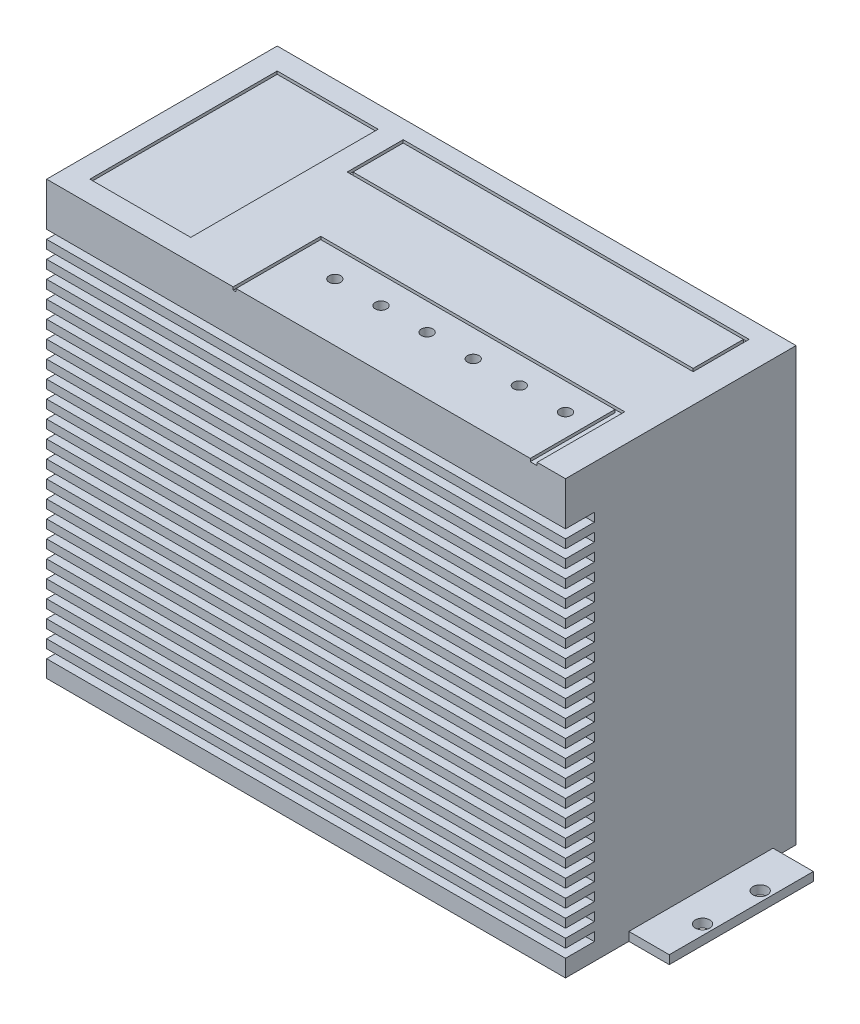
from build123d import *

# Parameters (mm, degrees)
SKETCH_1_W          = 180
SKETCH_1_H          = 150
EXTRUDE_1_DEPTH     = 40
CUT_EXTRUDE_1_REACH = 201.06
SKETCH_2_W          = 10
SKETCH_2_H          = 3
SKETCH_3_W          = 35
SKETCH_3_H          = 65
CUT_EXTRUDE_2_DEPTH = 1
SKETCH_4_W          = 120
SKETCH_4_H          = 19.42574098
SKETCH_4_W_2        = 118
SKETCH_4_H_2        = 17.42574098
CUT_EXTRUDE_3_DEPTH = 1
SKETCH_5_W          = 14
SKETCH_5_H          = 50
SKETCH_5_R          = 2.5
EXTRUDE_2_DEPTH     = 3
SKETCH_6_R          = 2
CUT_EXTRUDE_4_DEPTH = 4
CUT_EXTRUDE_5_DEPTH = 1


with BuildPart() as part:
    # 草图1 → 凸台-拉伸1 (new, symmetric)
    with BuildSketch(Plane.XY):
        Rectangle(SKETCH_1_W, SKETCH_1_H)
    extrude(amount=EXTRUDE_1_DEPTH, both=True)

    # 草图2 → 切除-拉伸1 (cut, up to next)
    with BuildSketch(Plane.ZY.offset(90), mode=Mode.PRIVATE) as cut_extrude_1_sk1:
        with Locations((35, 58.423056781)):
            Rectangle(SKETCH_2_W, SKETCH_2_H)
    cut_extrude_1_tool1 = extrude(cut_extrude_1_sk1.sketch, amount=-CUT_EXTRUDE_1_REACH, mode=Mode.PRIVATE) & part.part
    # 草图2 → 切除-拉伸1 (cut, up to next)
    with BuildSketch(Plane.ZY.offset(90), mode=Mode.PRIVATE) as cut_extrude_1_sk2:
        with Locations((35, 52.423056781)):
            Rectangle(SKETCH_2_W, SKETCH_2_H)
    cut_extrude_1_tool2 = extrude(cut_extrude_1_sk2.sketch, amount=-CUT_EXTRUDE_1_REACH, mode=Mode.PRIVATE) & part.part
    # 草图2 → 切除-拉伸1 (cut, up to next)
    with BuildSketch(Plane.ZY.offset(90), mode=Mode.PRIVATE) as cut_extrude_1_sk3:
        with Locations((35, 46.423056781)):
            Rectangle(SKETCH_2_W, SKETCH_2_H)
    cut_extrude_1_tool3 = extrude(cut_extrude_1_sk3.sketch, amount=-CUT_EXTRUDE_1_REACH, mode=Mode.PRIVATE) & part.part
    # 草图2 → 切除-拉伸1 (cut, up to next)
    with BuildSketch(Plane.ZY.offset(90), mode=Mode.PRIVATE) as cut_extrude_1_sk4:
        with Locations((35, 40.423056781)):
            Rectangle(SKETCH_2_W, SKETCH_2_H)
    cut_extrude_1_tool4 = extrude(cut_extrude_1_sk4.sketch, amount=-CUT_EXTRUDE_1_REACH, mode=Mode.PRIVATE) & part.part
    # 草图2 → 切除-拉伸1 (cut, up to next)
    with BuildSketch(Plane.ZY.offset(90), mode=Mode.PRIVATE) as cut_extrude_1_sk5:
        with Locations((35, 34.423056781)):
            Rectangle(SKETCH_2_W, SKETCH_2_H)
    cut_extrude_1_tool5 = extrude(cut_extrude_1_sk5.sketch, amount=-CUT_EXTRUDE_1_REACH, mode=Mode.PRIVATE) & part.part
    # 草图2 → 切除-拉伸1 (cut, up to next)
    with BuildSketch(Plane.ZY.offset(90), mode=Mode.PRIVATE) as cut_extrude_1_sk6:
        with Locations((35, 28.423056781)):
            Rectangle(SKETCH_2_W, SKETCH_2_H)
    cut_extrude_1_tool6 = extrude(cut_extrude_1_sk6.sketch, amount=-CUT_EXTRUDE_1_REACH, mode=Mode.PRIVATE) & part.part
    # 草图2 → 切除-拉伸1 (cut, up to next)
    with BuildSketch(Plane.ZY.offset(90), mode=Mode.PRIVATE) as cut_extrude_1_sk7:
        with Locations((35, 22.423056781)):
            Rectangle(SKETCH_2_W, SKETCH_2_H)
    cut_extrude_1_tool7 = extrude(cut_extrude_1_sk7.sketch, amount=-CUT_EXTRUDE_1_REACH, mode=Mode.PRIVATE) & part.part
    # 草图2 → 切除-拉伸1 (cut, up to next)
    with BuildSketch(Plane.ZY.offset(90), mode=Mode.PRIVATE) as cut_extrude_1_sk8:
        with Locations((35, 16.423056781)):
            Rectangle(SKETCH_2_W, SKETCH_2_H)
    cut_extrude_1_tool8 = extrude(cut_extrude_1_sk8.sketch, amount=-CUT_EXTRUDE_1_REACH, mode=Mode.PRIVATE) & part.part
    # 草图2 → 切除-拉伸1 (cut, up to next)
    with BuildSketch(Plane.ZY.offset(90), mode=Mode.PRIVATE) as cut_extrude_1_sk9:
        with Locations((35, 10.423056781)):
            Rectangle(SKETCH_2_W, SKETCH_2_H)
    cut_extrude_1_tool9 = extrude(cut_extrude_1_sk9.sketch, amount=-CUT_EXTRUDE_1_REACH, mode=Mode.PRIVATE) & part.part
    # 草图2 → 切除-拉伸1 (cut, up to next)
    with BuildSketch(Plane.ZY.offset(90), mode=Mode.PRIVATE) as cut_extrude_1_sk10:
        with Locations((35, 4.423056781)):
            Rectangle(SKETCH_2_W, SKETCH_2_H)
    cut_extrude_1_tool10 = extrude(cut_extrude_1_sk10.sketch, amount=-CUT_EXTRUDE_1_REACH, mode=Mode.PRIVATE) & part.part
    # 草图2 → 切除-拉伸1 (cut, up to next)
    with BuildSketch(Plane.ZY.offset(90), mode=Mode.PRIVATE) as cut_extrude_1_sk11:
        with Locations((35, -1.576943219)):
            Rectangle(SKETCH_2_W, SKETCH_2_H)
    cut_extrude_1_tool11 = extrude(cut_extrude_1_sk11.sketch, amount=-CUT_EXTRUDE_1_REACH, mode=Mode.PRIVATE) & part.part
    # 草图2 → 切除-拉伸1 (cut, up to next)
    with BuildSketch(Plane.ZY.offset(90), mode=Mode.PRIVATE) as cut_extrude_1_sk12:
        with Locations((35, -7.576943219)):
            Rectangle(SKETCH_2_W, SKETCH_2_H)
    cut_extrude_1_tool12 = extrude(cut_extrude_1_sk12.sketch, amount=-CUT_EXTRUDE_1_REACH, mode=Mode.PRIVATE) & part.part
    # 草图2 → 切除-拉伸1 (cut, up to next)
    with BuildSketch(Plane.ZY.offset(90), mode=Mode.PRIVATE) as cut_extrude_1_sk13:
        with Locations((35, -13.576943219)):
            Rectangle(SKETCH_2_W, SKETCH_2_H)
    cut_extrude_1_tool13 = extrude(cut_extrude_1_sk13.sketch, amount=-CUT_EXTRUDE_1_REACH, mode=Mode.PRIVATE) & part.part
    # 草图2 → 切除-拉伸1 (cut, up to next)
    with BuildSketch(Plane.ZY.offset(90), mode=Mode.PRIVATE) as cut_extrude_1_sk14:
        with Locations((35, -19.576943219)):
            Rectangle(SKETCH_2_W, SKETCH_2_H)
    cut_extrude_1_tool14 = extrude(cut_extrude_1_sk14.sketch, amount=-CUT_EXTRUDE_1_REACH, mode=Mode.PRIVATE) & part.part
    # 草图2 → 切除-拉伸1 (cut, up to next)
    with BuildSketch(Plane.ZY.offset(90), mode=Mode.PRIVATE) as cut_extrude_1_sk15:
        with Locations((35, -25.576943219)):
            Rectangle(SKETCH_2_W, SKETCH_2_H)
    cut_extrude_1_tool15 = extrude(cut_extrude_1_sk15.sketch, amount=-CUT_EXTRUDE_1_REACH, mode=Mode.PRIVATE) & part.part
    # 草图2 → 切除-拉伸1 (cut, up to next)
    with BuildSketch(Plane.ZY.offset(90), mode=Mode.PRIVATE) as cut_extrude_1_sk16:
        with Locations((35, -31.576943219)):
            Rectangle(SKETCH_2_W, SKETCH_2_H)
    cut_extrude_1_tool16 = extrude(cut_extrude_1_sk16.sketch, amount=-CUT_EXTRUDE_1_REACH, mode=Mode.PRIVATE) & part.part
    # 草图2 → 切除-拉伸1 (cut, up to next)
    with BuildSketch(Plane.ZY.offset(90), mode=Mode.PRIVATE) as cut_extrude_1_sk17:
        with Locations((35, -37.576943219)):
            Rectangle(SKETCH_2_W, SKETCH_2_H)
    cut_extrude_1_tool17 = extrude(cut_extrude_1_sk17.sketch, amount=-CUT_EXTRUDE_1_REACH, mode=Mode.PRIVATE) & part.part
    # 草图2 → 切除-拉伸1 (cut, up to next)
    with BuildSketch(Plane.ZY.offset(90), mode=Mode.PRIVATE) as cut_extrude_1_sk18:
        with Locations((35, -43.576943219)):
            Rectangle(SKETCH_2_W, SKETCH_2_H)
    cut_extrude_1_tool18 = extrude(cut_extrude_1_sk18.sketch, amount=-CUT_EXTRUDE_1_REACH, mode=Mode.PRIVATE) & part.part
    # 草图2 → 切除-拉伸1 (cut, up to next)
    with BuildSketch(Plane.ZY.offset(90), mode=Mode.PRIVATE) as cut_extrude_1_sk19:
        with Locations((35, -49.576943219)):
            Rectangle(SKETCH_2_W, SKETCH_2_H)
    cut_extrude_1_tool19 = extrude(cut_extrude_1_sk19.sketch, amount=-CUT_EXTRUDE_1_REACH, mode=Mode.PRIVATE) & part.part
    # 草图2 → 切除-拉伸1 (cut, up to next)
    with BuildSketch(Plane.ZY.offset(90), mode=Mode.PRIVATE) as cut_extrude_1_sk20:
        with Locations((35, -55.576943219)):
            Rectangle(SKETCH_2_W, SKETCH_2_H)
    cut_extrude_1_tool20 = extrude(cut_extrude_1_sk20.sketch, amount=-CUT_EXTRUDE_1_REACH, mode=Mode.PRIVATE) & part.part
    # 草图2 → 切除-拉伸1 (cut, up to next)
    with BuildSketch(Plane.ZY.offset(90), mode=Mode.PRIVATE) as cut_extrude_1_sk21:
        with Locations((35, -61.576943219)):
            Rectangle(SKETCH_2_W, SKETCH_2_H)
    cut_extrude_1_tool21 = extrude(cut_extrude_1_sk21.sketch, amount=-CUT_EXTRUDE_1_REACH, mode=Mode.PRIVATE) & part.part
    # 草图2 → 切除-拉伸1 (cut, up to next)
    with BuildSketch(Plane.ZY.offset(90), mode=Mode.PRIVATE) as cut_extrude_1_sk22:
        with Locations((35, -67.576943219)):
            Rectangle(SKETCH_2_W, SKETCH_2_H)
    cut_extrude_1_tool22 = extrude(cut_extrude_1_sk22.sketch, amount=-CUT_EXTRUDE_1_REACH, mode=Mode.PRIVATE) & part.part
    add(cut_extrude_1_tool1.solids().sort_by_distance((-90, 58.423057, 35))[0], mode=Mode.SUBTRACT)
    add(cut_extrude_1_tool2.solids().sort_by_distance((-90, 52.423057, 35))[0], mode=Mode.SUBTRACT)
    add(cut_extrude_1_tool3.solids().sort_by_distance((-90, 46.423057, 35))[0], mode=Mode.SUBTRACT)
    add(cut_extrude_1_tool4.solids().sort_by_distance((-90, 40.423057, 35))[0], mode=Mode.SUBTRACT)
    add(cut_extrude_1_tool5.solids().sort_by_distance((-90, 34.423057, 35))[0], mode=Mode.SUBTRACT)
    add(cut_extrude_1_tool6.solids().sort_by_distance((-90, 28.423057, 35))[0], mode=Mode.SUBTRACT)
    add(cut_extrude_1_tool7.solids().sort_by_distance((-90, 22.423057, 35))[0], mode=Mode.SUBTRACT)
    add(cut_extrude_1_tool8.solids().sort_by_distance((-90, 16.423057, 35))[0], mode=Mode.SUBTRACT)
    add(cut_extrude_1_tool9.solids().sort_by_distance((-90, 10.423057, 35))[0], mode=Mode.SUBTRACT)
    add(cut_extrude_1_tool10.solids().sort_by_distance((-90, 4.423057, 35))[0], mode=Mode.SUBTRACT)
    add(cut_extrude_1_tool11.solids().sort_by_distance((-90, -1.576943, 35))[0], mode=Mode.SUBTRACT)
    add(cut_extrude_1_tool12.solids().sort_by_distance((-90, -7.576943, 35))[0], mode=Mode.SUBTRACT)
    add(cut_extrude_1_tool13.solids().sort_by_distance((-90, -13.576943, 35))[0], mode=Mode.SUBTRACT)
    add(cut_extrude_1_tool14.solids().sort_by_distance((-90, -19.576943, 35))[0], mode=Mode.SUBTRACT)
    add(cut_extrude_1_tool15.solids().sort_by_distance((-90, -25.576943, 35))[0], mode=Mode.SUBTRACT)
    add(cut_extrude_1_tool16.solids().sort_by_distance((-90, -31.576943, 35))[0], mode=Mode.SUBTRACT)
    add(cut_extrude_1_tool17.solids().sort_by_distance((-90, -37.576943, 35))[0], mode=Mode.SUBTRACT)
    add(cut_extrude_1_tool18.solids().sort_by_distance((-90, -43.576943, 35))[0], mode=Mode.SUBTRACT)
    add(cut_extrude_1_tool19.solids().sort_by_distance((-90, -49.576943, 35))[0], mode=Mode.SUBTRACT)
    add(cut_extrude_1_tool20.solids().sort_by_distance((-90, -55.576943, 35))[0], mode=Mode.SUBTRACT)
    add(cut_extrude_1_tool21.solids().sort_by_distance((-90, -61.576943, 35))[0], mode=Mode.SUBTRACT)
    add(cut_extrude_1_tool22.solids().sort_by_distance((-90, -67.576943, 35))[0], mode=Mode.SUBTRACT)

    # 草图3 → 切除-拉伸2 (cut)
    with BuildSketch(Plane(origin=(0, 75, 0), x_dir=(1, 0, 0), z_dir=(0, 1, 0))):
        with Locations((-65, 0)):
            Rectangle(SKETCH_3_W, SKETCH_3_H)
    extrude(amount=-CUT_EXTRUDE_2_DEPTH, mode=Mode.SUBTRACT)

    # 草图4 → 切除-拉伸3 (cut)
    with BuildSketch(Plane(origin=(0, 75, 0), x_dir=(1, 0, 0), z_dir=(0, 1, 0))):
        with Locations((20, 24)):
            Rectangle(SKETCH_4_W, SKETCH_4_H)
        with Locations((20, 24)):
            Rectangle(SKETCH_4_W_2, SKETCH_4_H_2, mode=Mode.SUBTRACT)
    extrude(amount=-CUT_EXTRUDE_3_DEPTH, mode=Mode.SUBTRACT)

    # 草图5 → 凸台-拉伸2 (add)
    # profile 1 of 2: a face of its own
    with BuildSketch(Plane.XZ.offset(75)):
        with Locations((-97, -7)):
            Rectangle(SKETCH_5_W, SKETCH_5_H)
        with Locations((-100.540957797, 3)):
            Circle(SKETCH_5_R, mode=Mode.SUBTRACT)
        with Locations(Location((-100.540957797, -17, 0), (0, 0, 180))):
            Circle(SKETCH_5_R, mode=Mode.SUBTRACT)
    # profile 2 of 2: a face of its own
    with BuildSketch(Plane.XZ.offset(75)):
        with Locations((97, -7)):
            Rectangle(SKETCH_5_W, SKETCH_5_H)
        with Locations(Location((100.540957797, 3, 0), (0, 0, 180))):
            Circle(SKETCH_5_R, mode=Mode.SUBTRACT)
        with Locations((100.540957797, -17)):
            Circle(SKETCH_5_R, mode=Mode.SUBTRACT)
    extrude(amount=-EXTRUDE_2_DEPTH)

    # 草图6 → 切除-拉伸4 (cut)
    with BuildSketch(Plane(origin=(0, 75, 0), x_dir=(1, 0, 0), z_dir=(0, 1, 0))):
        with Locations(Location((-10, -20, 0), (0, 0, 180))):
            Circle(SKETCH_6_R)
        with Locations(Location((6, -20, 0), (0, 0, 180))):
            Circle(SKETCH_6_R)
        with Locations(Location((22, -20, 0), (0, 0, 180))):
            Circle(SKETCH_6_R)
        with Locations(Location((38, -20, 0), (0, 0, 180))):
            Circle(SKETCH_6_R)
        with Locations(Location((54, -20, 0), (0, 0, 180))):
            Circle(SKETCH_6_R)
        with Locations(Location((70, -20, 0), (0, 0, 180))):
            Circle(SKETCH_6_R)
    extrude(amount=-CUT_EXTRUDE_4_DEPTH, mode=Mode.SUBTRACT)

    # 草图7 → 切除-拉伸5 (cut)
    with BuildSketch(Plane(origin=(0, 75, 0), x_dir=(1, 0, 0), z_dir=(0, 1, 0))):
        Polygon((80.159624987, -9.614833725), (-25.279450467, -9.614833725), (-25.279450467, -40), (-24.279450467, -40), (-24.279450467, -10.614833725), (77.782924515, -10.614833725), (77.782924515, -40), (80.159624987, -40), align=None)
    extrude(amount=-CUT_EXTRUDE_5_DEPTH, mode=Mode.SUBTRACT)


solid = part.part
